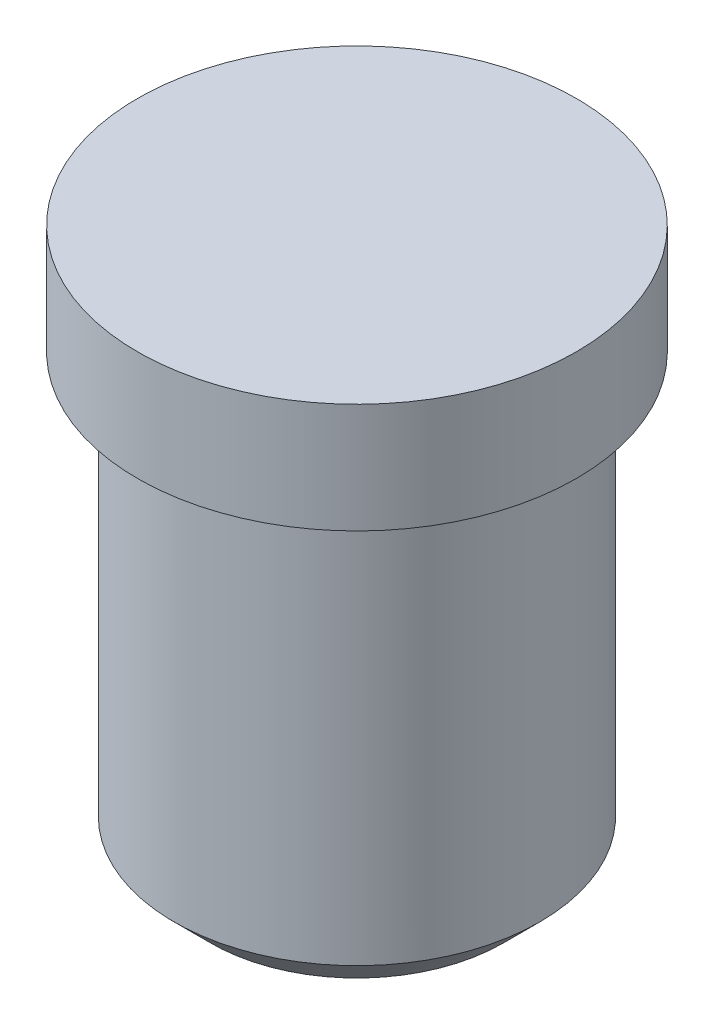
from build123d import *

# Parameters (mm, degrees)
CHAMFER1_SIZE = 1


with BuildPart() as part:
    # Sketch1 → Revolve1 (revolve)
    with BuildSketch(Plane.XY):
        Polygon((104.080767339, -426.85207641), (109.080767339, -426.85207641), (109.080767339, -414.85207641), (110.080767339, -414.85207641), (110.080767339, -411.85207641), (104.080767339, -411.85207641), align=None)
    revolve(axis=Axis((104.080767339, -427.306279578, 0), (0, 1, 0)))

    # Chamfer1
    chamfer1_edges = [part.edges().sort_by_distance(p)[0] for p in [
        (99.080767339, -426.85207641, 0),
    ]]
    chamfer(chamfer1_edges, length=CHAMFER1_SIZE)


solid = part.part
